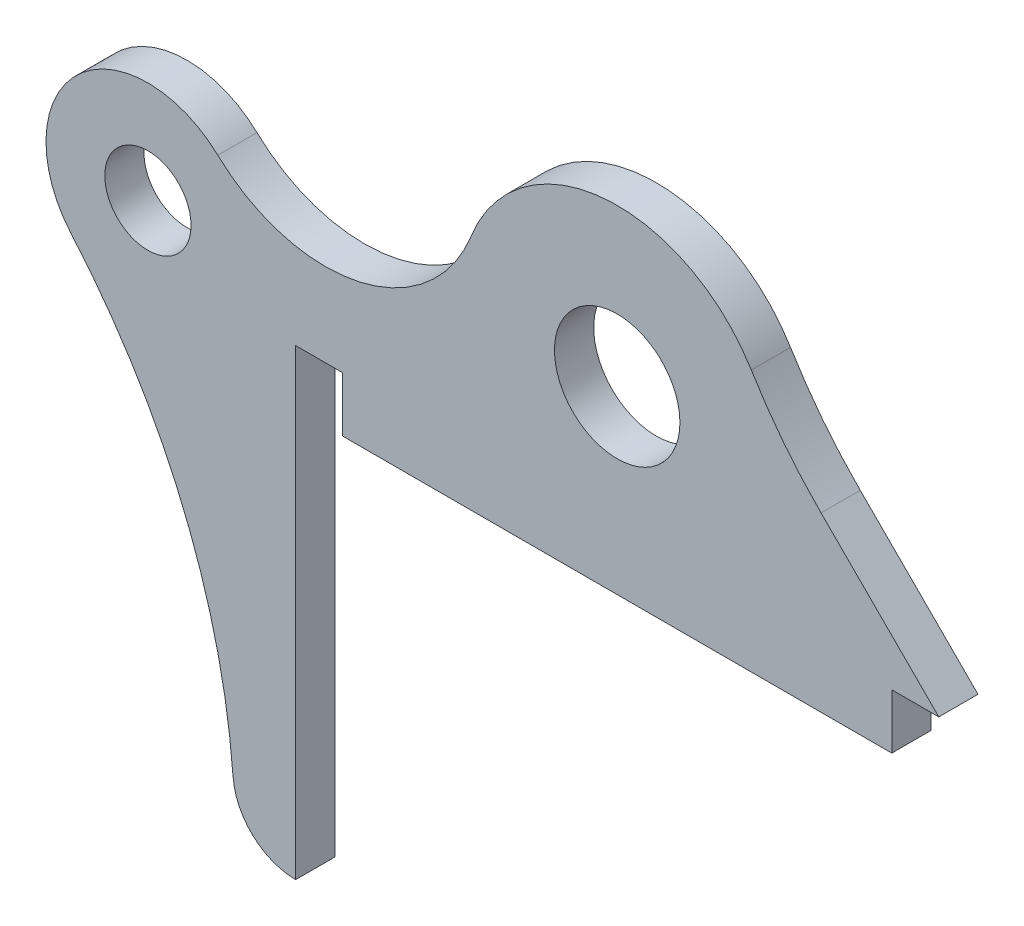
from build123d import *

# Parameters (mm, degrees)
SKETCH1_R           = 40
SKETCH1_R_2         = 27.5
BOSS_EXTRUDE1_DEPTH = 25


with BuildPart() as part:
    # Sketch1 → Boss-Extrude1 (new body)
    with BuildSketch(Plane.XY):
        with BuildLine():
            Line((-175.1, -115), (175.1, -115))
            Line((175.1, -115), (175.1, -80))
            Line((175.1, -80), (205.1, -80))
            Line((205.1, -80), (130.002057063, -4.902057063))
            ThreePointArc((130.002057063, -4.902057063), (106.058771733, 22.112599839), (85.533522855, 51.807494323))
            ThreePointArc((85.533522855, 51.807494323), (-8.510447338, 99.637203323), (-93.080630623, 36.551281821))
            ThreePointArc((-93.080630623, 36.551281821), (-164.286464639, -24.475575679), (-254.730193824, 0.313131132))
            ThreePointArc((-254.730193824, 0.313131132), (-344.272458908, -0.069434909), (-348.468561101, -89.514145872))
            ThreePointArc((-348.468561101, -89.514145872), (-276.775086195, -205.471406239), (-244.984042874, -338.043538078))
            ThreePointArc((-244.984042874, -338.043538078), (-232.286931391, -364.340599202), (-205.1, -375))
            Line((-205.1, -375), (-205.1, -80))
            Line((-205.1, -80), (-175.1, -80))
            Line((-175.1, -80), (-175.1, -115))
        make_face()
        Circle(SKETCH1_R, mode=Mode.SUBTRACT)
        with Locations((-299.3, -47)):
            Circle(SKETCH1_R_2, mode=Mode.SUBTRACT)
    extrude(amount=BOSS_EXTRUDE1_DEPTH)


solid = part.part
